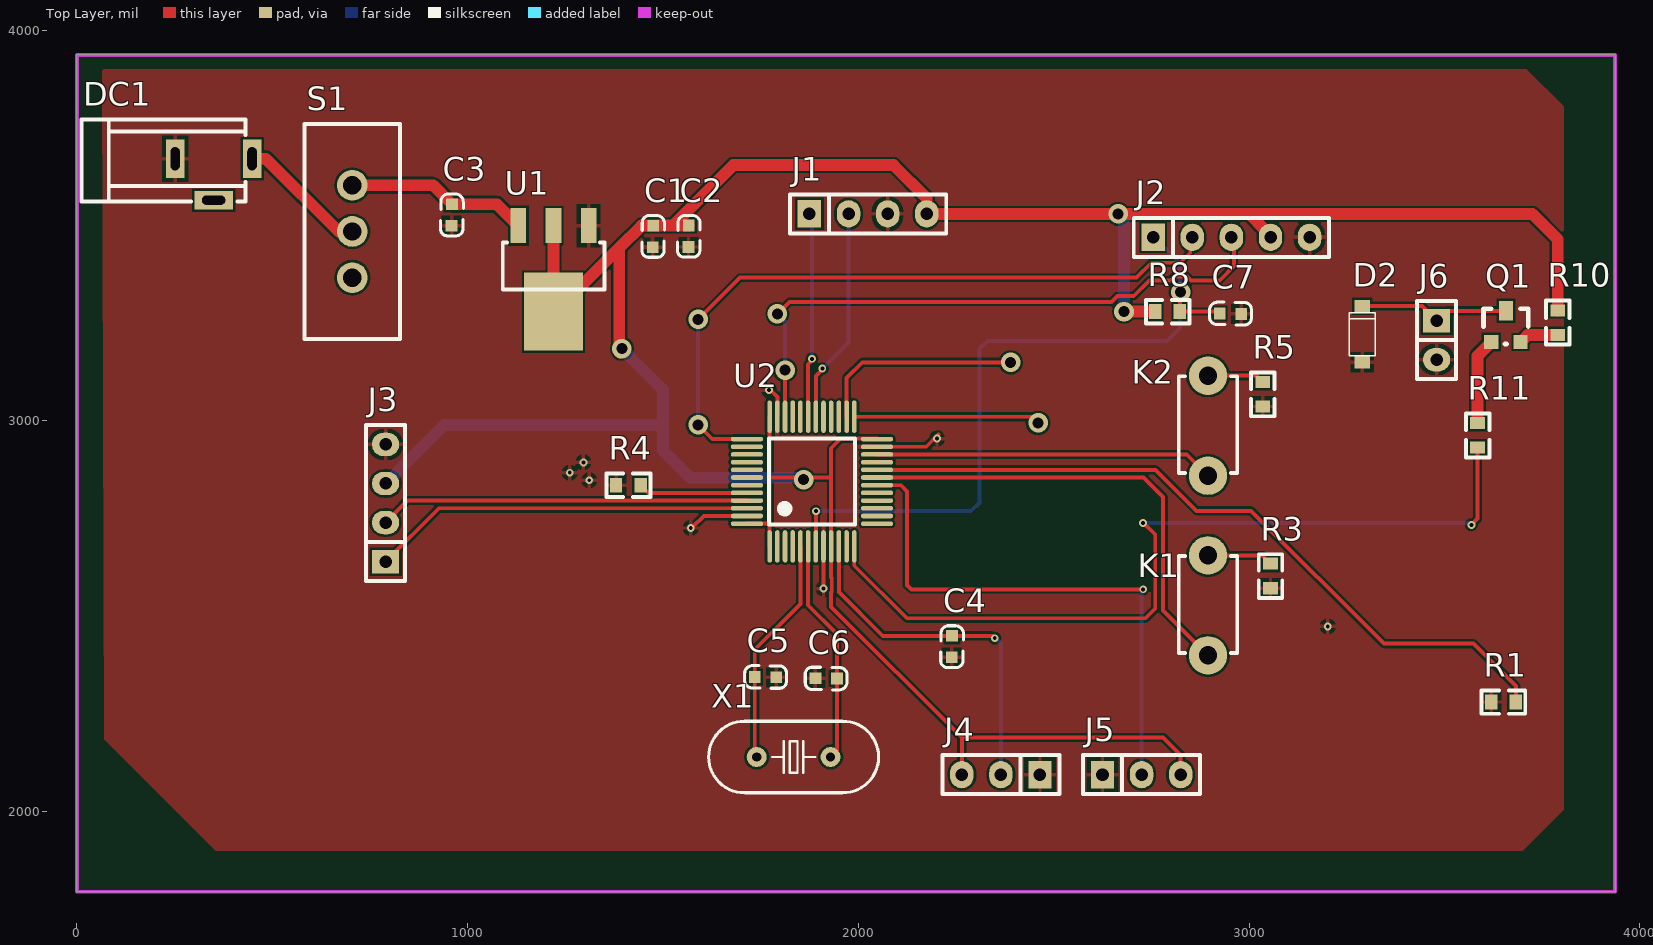
[diagram p0: Top Layer view]
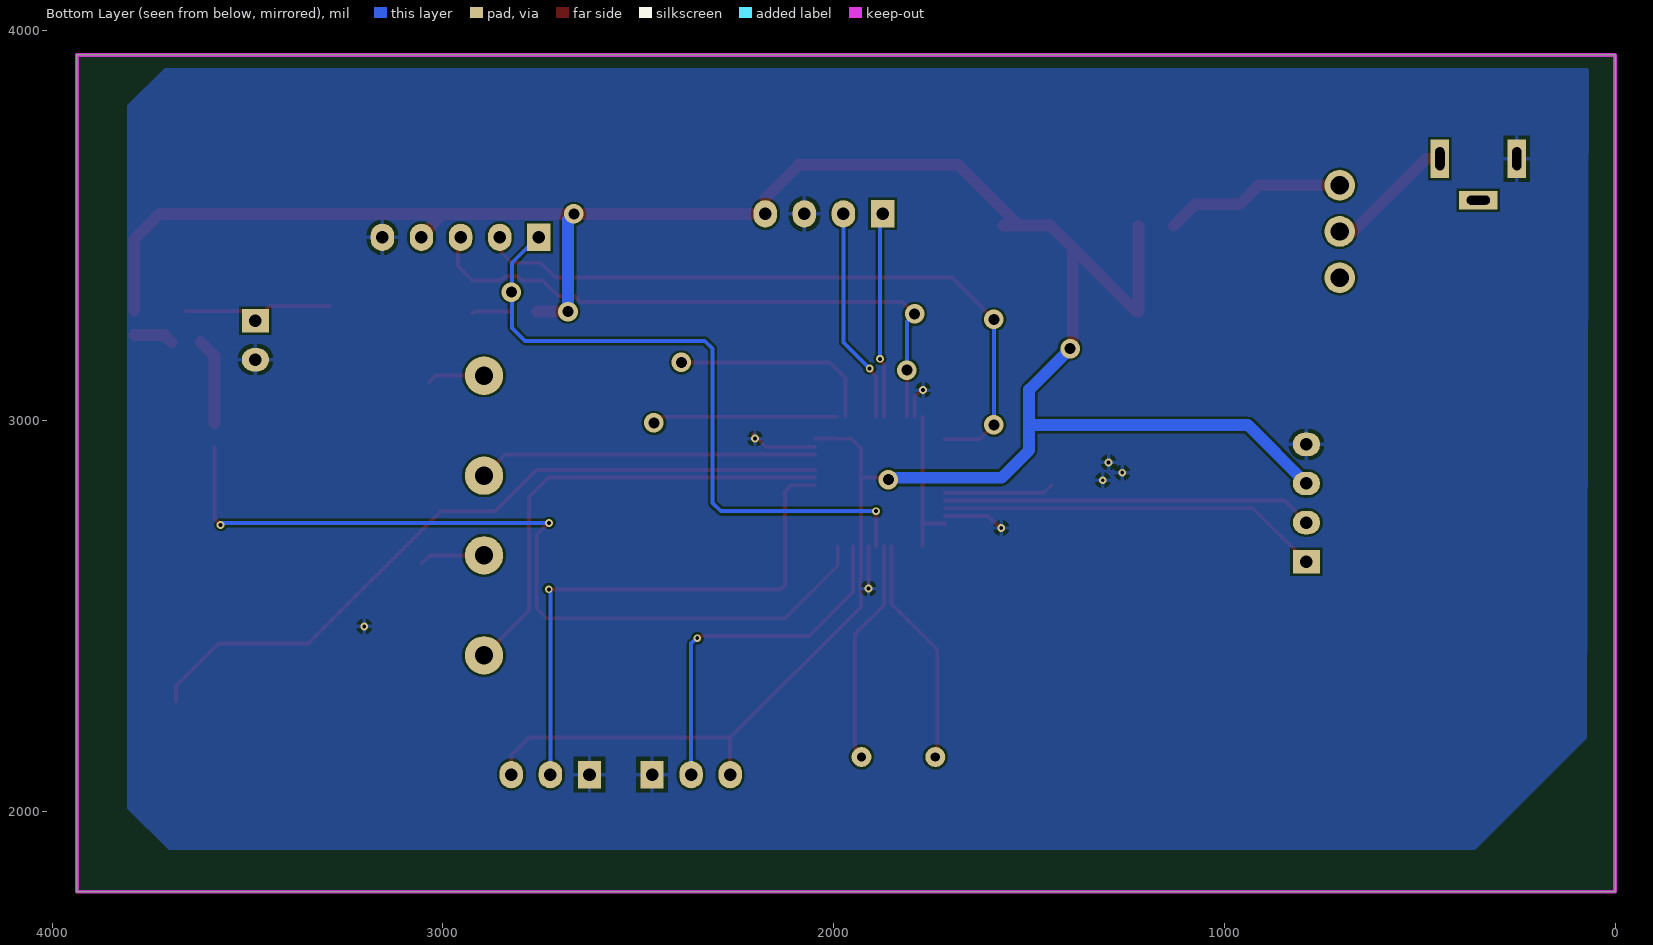
[diagram p1: Bottom Layer view, seen from below]
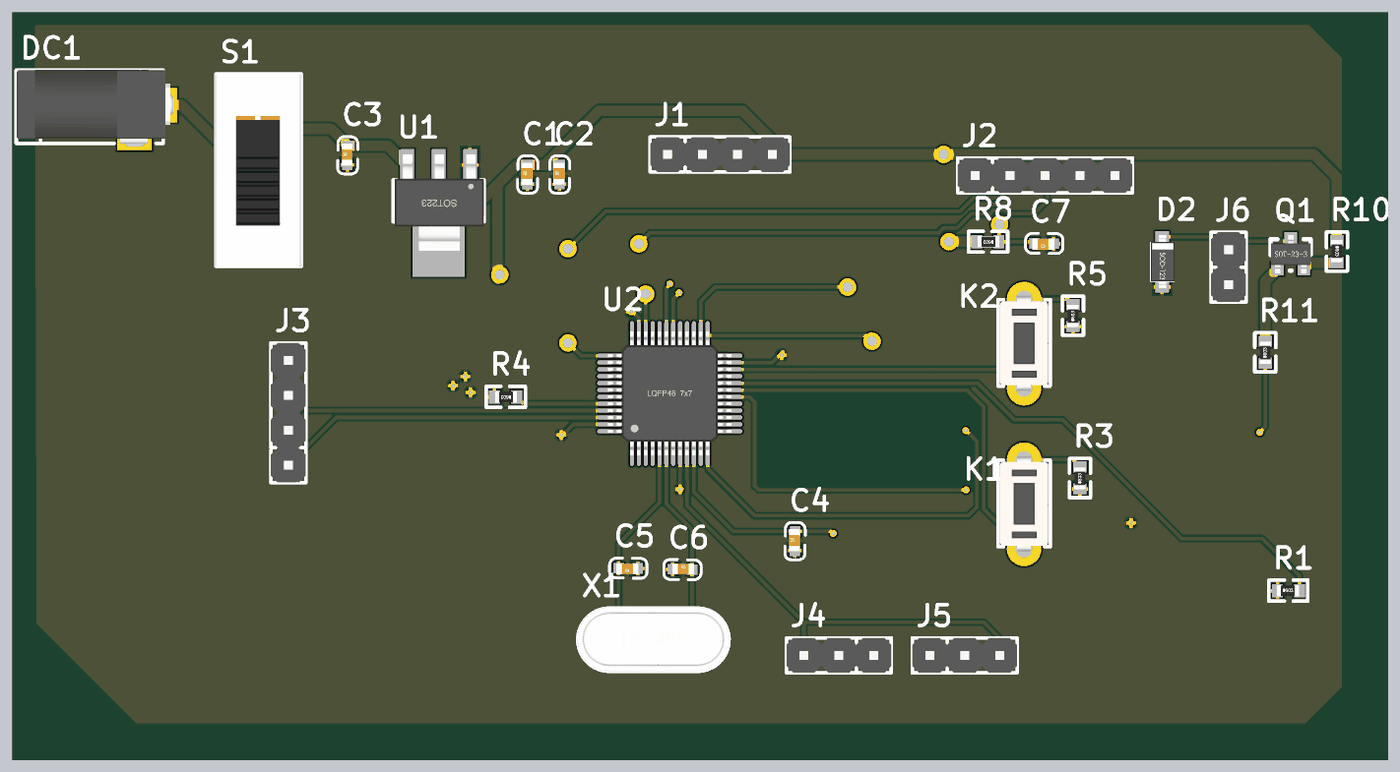
[diagram p2: 3D render of the assembled board from above, using the file's embedded part models]
# Altium PCB MISC82803.PcbDoc
Units mil, origin at the board's own origin, x right, y up, seen from the top; angles counter-clockwise.
Board outline 3937.01 x 2142.01 mil, 2 copper layers (Top Layer, Bottom Layer); 29 components, 25 nets, 118 pads, 26 vias.

## Layer stack, top to bottom (the 12.6 mil dielectric is the usual default, probably not edited)
Top Solder: solder mask 0.4, Solder Resist, Dk 3.5
Top Layer: signal copper 1.4
Dielectric 1: dielectric 12.6, FR-4, Dk 4.8
Bottom Layer: signal copper 1.4
Bottom Solder: solder mask 0.4, Solder Resist, Dk 3.5

## Board outline
0,1795 3937.01,1795 3937.01,3937.01 0,3937.01

## Design rules (kind name [scope] priority, off if disabled: settings)
Clearance [All] p1: gap=6 ignorepadtopadclearanceinfootprint=FALSE
PolygonConnect [All] p1: connectstyle=Relief reliefconductorwidth=10 reliefentries=4 polygonreliefangle="90 Angle" airgapwidth=10
RoutingVias [All] p1: holewidth=10 width=20 viastyle="Through Hole" minholewidth=10 minwidth=20 maxholewidth=10 maxwidth=50
SolderMaskExpansion [All] p1: expansion=4
Width [All] p1: maxlimit=50 minlimit=10 preferedwidth=10
30 further rules are at their usual default settings.

## Components (designator, comment, footprint, x,y, rotation, side; value= is the part's Value field where it differs from the comment)
C1 "10uF" 0603C 1473.65,3444.79 r90 top
C2 "0.1uF" 0603C 1565,3445 r90 top
C3 "10uF" 0603C 958.65,3499.79 r90 top
C4 "0.1uF" 0603C 2238.65,2394.79 r90 top
C5 "20pF" 0603C 1790.21,2343.65 r180 top
C6 "20pF" 0603C 1890,2342.01 r0 top
C7 "0.1uF" 0603C 2980.21,3273.65 r180 top
D2 "DIODE" SOD-123 3290,3152.01 r90 top
DC1 "DC_Socket" DC-002 448.43,3671.3 r180 top
J1 "Pin HDR1X4" "Pin HDR1X4/2.54mm-S" 1875,3530 r90 top
J2 "Pin HDR1X5" "Pin HDR1X5/2.54mm-S" 2755,3470 r90 top
J3 "Pin HDR1X4" "Pin HDR1X4/2.54mm-S" 790,2640 r180 top
J4 "Pin HDR1X3" "Pin HDR1X3/2.54mm-S" 2465,2095 r270 top
J5 "Pin HDR1X3" "Pin HDR1X3/2.54mm-S" 2625,2095 r90 top
J6 "Pin HDR1X2" "Pin HDR1X2/2.54mm-S" 3480,3257.01 r0 top
K1 "KEY" DIP-3X6X4.3 2895,2400 r90 top
K2 "KEY" DIP-3X6X4.3 2895,2860 r90 top
Q1 "PNP" SOT-23 3655,3237.01 r0 top
R1 "10K" 0603R 3620,2280.65 r0 top
R3 "10K" 0603R 3055,2572.01 r90 top
R4 "10K" 0603R 1442.99,2835.63 r180 top
R5 "10K" 0603R 3035,3037.01 r90 top
R8 "10K" 0603R 2822.99,3280 r180 top
R10 "470" 0603R 3790,3282.99 r270 top
R11 "470" 0603R 3585,2932.01 r90 top
S1 "SS-12D10" SS-12D10 705,3603.11 r270 top
U1 "AMS1117" SOT223 1220,3500 r180 top
U2 "STM32F103C8T6" "LQFP48 7X7" 1881.42,2845.47 r0 top
X1 "XTAL-2P" "OSC HC-49S" 1834.49,2140 r0 top

## Footprints (in the part's own frame and the unit in brackets; to place one, negate y for a bottom-side part, rotate by r counter-clockwise, add the part's x,y. Pads: shape width x height; smd on the part's side, far side on the other; paste and mask are expansions set on the pad)
0603C [mil]
  rect 30x30 smd: 1(0.21,-0.35) 2(55.21,-1.35)
  silkscreen extent -26,-30 81,28, body extent -1,-15 62,17, height 12
0603R [mm]
  rect 0.8x0.965 smd: 1(0,0) 2(1.6,0)
  silkscreen extent -0.64,-0.76 2.21,0.76, body extent -0.04,-0.41 1.56,0.41, height 0.45
DC-002 [mm] "3.5X1.1mm"
  rect 1.2x2.5 hole 0.6 slot 1.5 at 90 deg: 1(0,0) 2(5,0)
  rect 2.5x1.2 hole 0.6 slot 1.5 at 0 deg: 3(2.5,2.7)
  silkscreen extent 0.43,-2.54 11.1,2.79, body extent -0.25,-2.55 11.05,2.8, height 7.3
DIP-3X6X4.3 [mm]
  round 2.5 hole 1.2: 1(0,0) 3(6.5,0)
  silkscreen extent 0.16,-1.9 6.46,1.9, body extent -0.64,-1.75 7.19,1.75, height 4.31
"LQFP48 7X7" [mm]
  oval 0.3x2.1 smd: 1(-2.75,-4.227) 2(-2.25,-4.227) 3(-1.75,-4.227) 4(-1.25,-4.227) 5(-0.75,-4.227) 6(-0.25,-4.227) 7(0.25,-4.227) 8(0.75,-4.227) 9(1.25,-4.227) 10(1.75,-4.227) 11(2.25,-4.227) 12(2.75,-4.227) 25(2.75,4.202) 26(2.25,4.202) 27(1.75,4.202) 28(1.25,4.202) 29(0.75,4.202) 30(0.25,4.202) 31(-0.25,4.202) 32(-0.75,4.202) 33(-1.25,4.202) 34(-1.75,4.202) 35(-2.25,4.202) 36(-2.75,4.202)
  oval 2.1x0.3 smd: 13(4.227,-2.75) 14(4.227,-2.25) 15(4.227,-1.75) 16(4.227,-1.25) 17(4.227,-0.75) 18(4.227,-0.25) 19(4.227,0.25) 20(4.227,0.75) 21(4.227,1.25) 22(4.227,1.75) 23(4.227,2.25) 24(4.227,2.75) 37(-4.227,2.75) 38(-4.227,2.25) 39(-4.227,1.75) 40(-4.227,1.25) 41(-4.227,0.75) 42(-4.227,0.25) 43(-4.227,-0.25) 44(-4.227,-0.75) 45(-4.227,-1.25) 46(-4.227,-1.75) 47(-4.227,-2.25) 48(-4.227,-2.75)
  silkscreen extent -2.79,-2.79 2.79,2.79, body extent -4.51,-4.5 4.5,4.5, height 1.45
"OSC HC-49S" [mm]
  round 1.3 hole 0.6: 1(-2.4,0) 2(2.4,0)
  silkscreen extent -5.52,-2.32 5.52,2.33, body extent -5.53,-2.29 5.53,2.36, height 4.13
"Pin HDR1X2/2.54mm-S" [mil]
  rect 70x60 hole 32: 1(0,0)
  oval 70x60 hole 32: 2(0,-100)
  silkscreen extent -50,-150 50,50, body extent -50,-150 50,50, height 336
"Pin HDR1X3/2.54mm-S" [mil]
  rect 70x60 hole 32: 1(0,0)
  oval 70x60 hole 32: 2(0,-100) 3(0,-200)
  silkscreen extent -50,-250 50,50, body extent -50,-250 50,50, height 336
"Pin HDR1X4/2.54mm-S" [mil]
  rect 70x60 hole 32: 1(0,0)
  oval 70x60 hole 32: 2(0,-100) 3(0,-200) 4(0,-300)
  silkscreen extent -50,-350 50,50, body extent -50,-350 50,50, height 336
"Pin HDR1X5/2.54mm-S" [mil]
  rect 70x60 hole 32: 1(0,0)
  oval 70x60 hole 32: 2(0,-100) 3(0,-200) 4(0,-300) 5(0,-400)
  silkscreen extent -50,-450 50,50, body extent -50,-450 50,50, height 336
SOD-123 [mm] "塑封二极管"
  rect 0.8x1 smd: A(-0.051,0) K(3.607,0)
  silkscreen extent 0.38,-0.85 3.18,0.85, body extent -0.12,-0.89 3.73,0.81, height 1.43
SOT223 [mil]
  rect 40x90 smd: 1(-90,0) 2(0,0) 3(90,0)
  rect 150x200 smd: 2(0,220)
  silkscreen extent -130,43 130,163, body extent -130,-30 126,246, height 65
SOT-23 [mil]
  rect 36x36 smd: B(-35,-35) E(40,-35)
  rect 36x50 smd: C(3,45)
  silkscreen extent -55,-40 60,50, body extent -54,-48 60,62, height 47
SS-12D10 [mm]
  round 2 hole 1.2: 1(0,0) 2(3,0) 3(6,0)
  silkscreen extent -4,-3.1 10,3.1, body extent -3.95,-3.15 10.05,3.05, height 9.65

## Part data
C1 C2 C3 C4 C5 C6 C7: library part CAP, "Non-polar capacitor"
D2: "General diode"
Q1: "PNP transistor"
R1 R3 R4 R5 R8 R10 R11: library part RES
U1: "Three-terminal voltage regulator"
X1: "2-pin passive crystal oscillator"

## Via types
v1: diameter 20, hole 10, Top Layer to Bottom Layer, 15 vias
v2: diameter 50, hole 28, Top Layer to Bottom Layer, 11 vias

## Nets (pads, with @x,y where several pads share a name; then routed paths per layer and width w, separated by ;. In a path a pad name is that pad's centre, name@x,y a point inside that pad or via, vN(x,y) a via of type N, cw(c..) or ccw(c..) an arc to the next point about the centre after c; other vN are vias at no path point)
+5: C3.2 S1.1 U1.3 | length 467.7
  Top Layer w30: S1.1 911.89,3603.11 C3.2 1075,3555 U1.3
adc1: C4.2 J4.2 U2.10 | length 920.8
  Top Layer w10: U2.10 1950.32,2562.23 2062.54,2450 C4.2 2343.27,2450 v1(2349.14,2444.14)
  Bottom Layer w10: v1@2350,2445 2365,2430 J4.2
boot: R4.1 U2.44 | length 280.2
  Top Layer w10: R4.1 1462.68,2815.95 U2.44
GND: C1.1 C2.1 C3.1 C4.1 C5.1 C6.1 C7.1 D2.A DC1.2 J1.3 J2.5 J3.4 J4.1 J5.1 J6.2 R1.1 R3.1 R4.2 R5.1 U1.1 U2.8 U2.23 U2.35 U2.47 | length 507.4
  Top Layer w10: v1@1574.76,2727.04 1604.6,2756.89 U2.47 ; v1@1774.67,3080 1792.83,3061.84 U2.35 ; v1(1910.94,2570.93) U2.8 ; U2.23 2173.85,2934.06 2205,2965.21
  other v1: 3201.42,2474.14 1571.17,2726.18 1311.42,2848.25 1261.42,2867.67 1296.42,2894.14 2201.42,2955.04 1771.09,3079.14
ir_ext: J5.2 U2.18 | length 1410.6
  Top Layer w10: U2.18 2109.37,2835.63 2125,2820 2124.14,2819.14 2124.14,2579.14 ; 2125,2580 2135.86,2569.14 v1(2729.14,2569.14)
  Bottom Layer w10: J5.2 2725,2565 v1(2729.14,2569.14) v1@2730,2570
mcu_key1: K1.1 U2.19 | length 1206
  Top Layer w10: U2.19 2730.31,2855.32 2780.16,2805.47 2780.16,2514.84 K1.1
mcu_key2: K2.1 U2.22 | length 869.7
  Top Layer w10: U2.22 2840.63,2914.37 K2.1
NetD2_K: D2.K J6.1 Q1.C | length 393.7
  Top Layer w10: D2.K 3443,3294.01 J6.1 3505,3282.01 Q1.C
NetDC1_1: DC1.1 S1.2 | length 333.7
  Top Layer w30: DC1.1 483.7,3671.3 670,3485 S1.2
NetK1_3: K1.3 R3.2 | length 169.2
  Top Layer w10: K1.3 3035,2655.91 3035,2655 R3.2
NetK2_3: K2.3 R5.2 | length 146.6
  Top Layer w10: K2.3 3019.09,3115.91 R5.2
NetQ1_B: Q1.B R11.2 | length 221.5
  Top Layer w30: R11.2 3585,3167.01 Q1.B
NetQ1_E: Q1.E R10.2 | length 102.5
  Top Layer w30: Q1.E 3712.99,3220 R10.2
NetR1_2: R1.2 U2.20 | length 1904.2
  Top Layer w10: U2.20 2760.95,2875 2865.95,2770 3005,2770 3345,2430 3575,2430 3682.99,2322.01 R1.2@3682.99,2282.01
nrst: C7.2 J2.1 R8.1 U2.7 | length 1866.5
  Top Layer w10: U2.7 1891.26,2766.26 v1@1895,2770 ; v2(2825,3330) 2822.99,3327.99 R8.1 2920,3280 C7.2
  Bottom Layer w10: v1(1891.42,2769.14) 2289.14,2769.14 2310,2790 2310,3185 2330,3205 2790,3205 2822.99,3237.99 2822.99,3405 2757.99,3470 J2.1
oled_scl: J3.2 U2.45 | length 948.3
  Top Layer w10: J3.2 846.26,2796.26 U2.45
oled_sda: J3.1 U2.46 | length 981.6
  Top Layer w10: J3.1 926.57,2776.57 U2.46
osc_in: C5.2 U2.5 X1.1 | length 589.5
  Top Layer w10: X1.1 1735,2145 C5.2 1735,2415 1851.89,2531.89 U2.5
osc_out: C6.2 U2.6 X1.2 | length 576.3
  Top Layer w10: U2.6 1871.57,2528.43 1945.21,2454.79 C6.2 1945.21,2156.24 X1.2
pwm: R11.1 U2.12 | length 2166.6
  Top Layer w10: U2.12 1989.69,2629.45 2124.14,2495 2735,2495 2760,2520 2760,2709.14 v1@2729.14,2740 ; v1(3569.14,2734.14) 3585,2750 R11.1
  Bottom Layer w10: v1(2728.27,2739.14) 3565.86,2739.14 v1@3570,2735
swclk: J2.2 U2.37 | length 1781.9
  Top Layer w10: v2(1590,2990) 1626.26,2953.74 U2.37 ; v2(1590,3260) 1696.89,3366.89 2711.89,3366.89 2750,3405 2824.05,3405 2849.52,3430.48 2849.52,3464.52 J2.2
  Bottom Layer w10: v2(1590,2990) v2(1590,3260)
swdio: J2.3 U2.34 | length 1567.4
  Top Layer w10: v2(1792.83,3274) 1823.83,3305 2648.43,3305 2663.43,3320 2705,3320 2745,3360 2798.43,3360 2808.43,3370 2841.57,3370 2851.57,3360 2925,3360 2961.26,3396.26 J2.3@2961.26,3465 ; U2.34 v2(1812.52,3130)
  Bottom Layer w10: v2(1792.83,3274) 1812.52,3254.31 v2(1812.52,3130)
uart_spk_rx: J1.1 U2.31 | length 521.7
  Top Layer w10: U2.31 1871.57,3145.16 v1@1881.42,3155
  Bottom Layer w10: J1.1 1881.42,3523.58 v1(1881.42,3159.14)
uart_spk_tx: J1.2 U2.30 | length 556.1
  Top Layer w10: U2.30 1891.26,3114.79 v1@1911.47,3135
  Bottom Layer w10: v1(1907.89,3134.14) 1975,3201.25 J1.2
VCC: C1.2 C2.2 J1.4 J2.4 J3.3 J4.3 J5.3 R8.2 R10.1 U1.2 U2.1 U2.9 U2.24 U2.36 U2.48 | length 7690
  Top Layer w10: U2.48 1770.35,2737.2 1773.15,2740 ; U2.1 1773.15,2740 ; U2.36 1773.15,2855 ; U2.24@2047.83,2954.96 1998.76,2954.96 1998.35,2954.55 1954.87,2954.55 1930.63,2930.31 1930.63,2855 ; J4.3 2265,2190 ; J5.3 2825,2145 2780,2190 2265,2190 ; 1773.15,2740 1773.15,2855 ; 1773.15,2855 1930.63,2855 ; 1930.63,2855 U2.9 1930.63,2599.37 1931.94,2598.06 1931.94,2562.23 1930.63,2560.91 1930.63,2524.37 2265,2190
  Top Layer w30: U1.2@1220,3500 1220,3280 1225,3280 1388.44,3443.44 ; v2@1390,3174.96 1388.44,3176.52 1388.44,3443.44 ; C2.2 1525,3500.21 ; v2(2680,3280) R8.2 ; J2.4@3040,3465 3040,3490 3000,3530 ; R10.1 3790,3465 3725,3530 3000,3530 ; 1388.44,3443.44 1445.21,3500.21 1525,3500.21 ; 1525,3500.21 1679.79,3655 2090,3655 2175,3570 J1.4 v2(2665,3530) 3000,3530
  Bottom Layer w30: J3.3 940,2990 1500,2990 ; v2(1395,3185.3) 1500,3080.3 1500,2990 ; v2@1847.82,2855 1570,2855 1500,2925 1500,2990 ; v2(2665,3530) 2680,3515 v2(2680,3280)
  other v2: 1860,2850
pads on no net: DC1.3 S1.3 U2.2 U2.3 U2.4 U2.11 U2.13 U2.14 U2.15 U2.16 U2.17 U2.21 U2.25 U2.26 U2.27 U2.28 U2.29 U2.32 U2.33 U2.38 U2.39 U2.40 U2.41 U2.42 U2.43
copper on no net: | length 1026.7
  Top Layer w10: 1970,3010.89 1970,3110 2010,3150 v2(2390,3150) ; 1989.69,3010.89 2444.11,3010.89 v2(2460,2995)
  Bottom Layer w10: v2@2380,3140 v2(2390,3150)

## Polygon pours and split planes (outlines as drawn)
GND on Top Layer (solid, remove dead copper, pour order 6): 65,3900 3710,3900 3805,3805 3805,2005 3700,1900 355,1900 70,2185
GND on Bottom Layer (solid, remove dead copper, pour order 8): 67.5,3902.5 3712.5,3902.5 3807.5,3807.5 3807.5,2007.5 3702.5,1902.5 357.5,1902.5 72.5,2187.5

## Keep-outs
Keep-Out Layer:
  the board outline again, w10